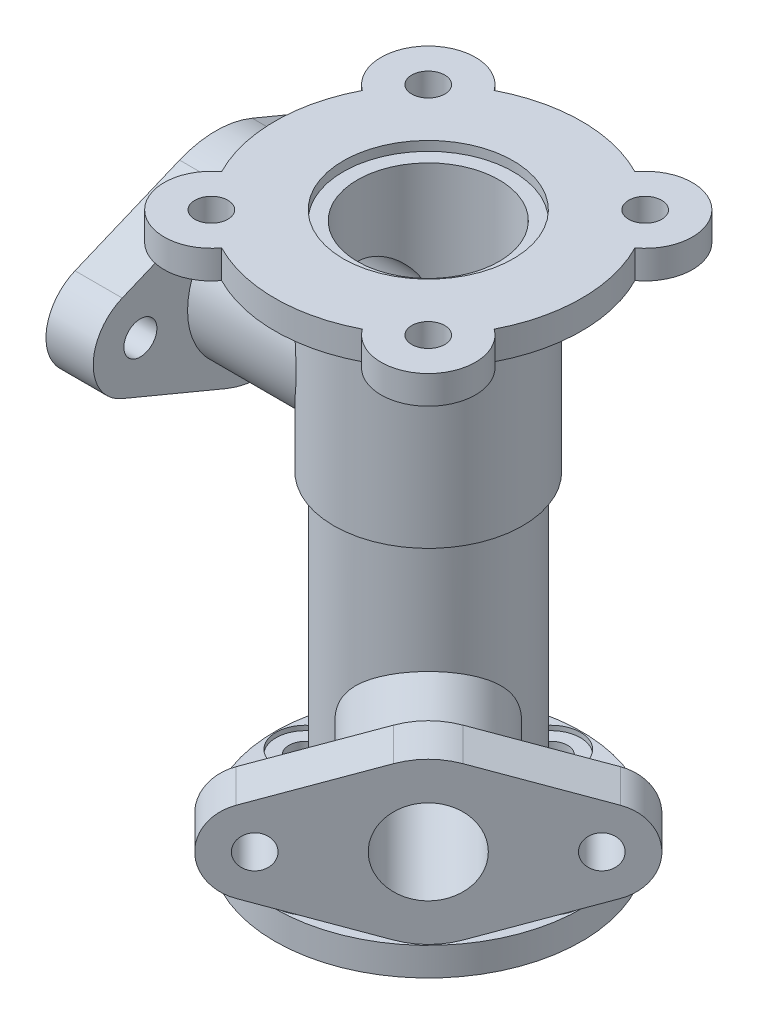
from build123d import *

# Parameters (mm, degrees)
SKETCH1_R           = 32.5
BOSS_EXTRUDE1_DEPTH = 6
SKETCH2_R           = 18
BOSS_EXTRUDE2_DEPTH = 64
SKETCH3_R           = 20
BOSS_EXTRUDE3_DEPTH = 48
BOSS_EXTRUDE4_START = -6
SKETCH4_R           = 32.5
SKETCH4_R_2         = 10
SKETCH4_R_3         = 20
BOSS_EXTRUDE4_DEPTH = 6
SKETCH5_R           = 16
BOSS_EXTRUDE5_DEPTH = 45
BOSS_EXTRUDE6_DEPTH = 10
SKETCH8_R           = 14
BOSS_EXTRUDE7_DEPTH = 45
BOSS_EXTRUDE8_DEPTH = 10
SKETCH10_R          = 13
CUT_EXTRUDE1_DEPTH  = 70
SKETCH11_R          = 9
CUT_EXTRUDE2_DEPTH  = 45
SKETCH12_R          = 11
CUT_EXTRUDE3_DEPTH  = 45
CUT_EXTRUDE4_START  = -2
SKETCH13_R          = 18
CUT_EXTRUDE4_DEPTH  = 2
SKETCH14_R          = 15
CUT_EXTRUDE5_DEPTH  = 36
SKETCH15_R          = 14
CUT_EXTRUDE6_DEPTH  = 3
SKETCH16_R          = 3.5
CUT_EXTRUDE7_DEPTH  = 20
SKETCH17_R          = 6.5
CUT_EXTRUDE8_DEPTH  = 1
SKETCH18_R          = 3.5
CUT_EXTRUDE9_DEPTH  = 10
SKETCH19_R          = 3.5
CUT_EXTRUDE10_DEPTH = 10
SKETCH20_R          = 3.5
CUT_EXTRUDE11_DEPTH = 20
SKETCH21_R          = 6.25
CUT_EXTRUDE12_DEPTH = 1
SKETCH22_R          = 10
CUT_EXTRUDE13_DEPTH = 50


with BuildPart() as part:
    # Sketch1 → Boss-Extrude1 (new body)
    with BuildSketch(Plane(origin=(0, 0, 0), x_dir=(1, 0, 0), z_dir=(0, 1, 0))):
        with Locations(Location((0, 0, 0), (0, 0, 270))):
            Circle(SKETCH1_R)
    extrude(amount=BOSS_EXTRUDE1_DEPTH)

    # Sketch2 → Boss-Extrude2 (add)
    with BuildSketch(Plane(origin=(0, 6, 0), x_dir=(1, 0, 0), z_dir=(0, 1, 0))):
        with Locations(Location((0, 0, 0), (0, 0, 270))):
            Circle(SKETCH2_R)
    extrude(amount=BOSS_EXTRUDE2_DEPTH)

    # Sketch3 → Boss-Extrude3 (add)
    with BuildSketch(Plane(origin=(0, 70, 0), x_dir=(1, 0, 0), z_dir=(0, 1, 0))):
        with Locations(Location((0, 0, 0), (0, 0, 270))):
            Circle(SKETCH3_R)
    extrude(amount=BOSS_EXTRUDE3_DEPTH)

    # Sketch4 → Boss-Extrude4 (add)
    # profile 1 of 18: a face of its own
    with BuildSketch(Plane(origin=(0, 118, 0), x_dir=(1, 0, 0), z_dir=(0, 1, 0)).offset(BOSS_EXTRUDE4_START)):
        with Locations(Location((0, 0, 0), (0, 0, 270))):
            Circle(SKETCH4_R)
    # profile 2 of 18: a face of its own
    with BuildSketch(Plane(origin=(0, 118, 0), x_dir=(1, 0, 0), z_dir=(0, 1, 0)).offset(BOSS_EXTRUDE4_START)):
        with Locations((22.980970389, 22.980970389)):
            Circle(SKETCH4_R_2)
    # profile 3 of 18: a face of its own
    with BuildSketch(Plane(origin=(0, 118, 0), x_dir=(1, 0, 0), z_dir=(0, 1, 0)).offset(BOSS_EXTRUDE4_START)):
        with Locations(Location((0, 0, 0), (0, 0, 270))):
            Circle(SKETCH4_R)
    # profile 4 of 18: a face of its own
    with BuildSketch(Plane(origin=(0, 118, 0), x_dir=(1, 0, 0), z_dir=(0, 1, 0)).offset(BOSS_EXTRUDE4_START)):
        with Locations((22.980970389, 22.980970389)):
            Circle(SKETCH4_R_2)
    # profile 5 of 18: a face of its own
    with BuildSketch(Plane(origin=(0, 118, 0), x_dir=(1, 0, 0), z_dir=(0, 1, 0)).offset(BOSS_EXTRUDE4_START)):
        with Locations((-22.980970389, 22.980970389)):
            Circle(SKETCH4_R_2)
    # profile 6 of 18: a face of its own
    with BuildSketch(Plane(origin=(0, 118, 0), x_dir=(1, 0, 0), z_dir=(0, 1, 0)).offset(BOSS_EXTRUDE4_START)):
        with Locations(Location((0, 0, 0), (0, 0, 270))):
            Circle(SKETCH4_R)
        with Locations(Location((0, 0, 0), (0, 0, 270))):
            Circle(SKETCH4_R_3, mode=Mode.SUBTRACT)
    # profile 7 of 18: a face of its own
    with BuildSketch(Plane(origin=(0, 118, 0), x_dir=(1, 0, 0), z_dir=(0, 1, 0)).offset(BOSS_EXTRUDE4_START)):
        with Locations((-22.980970389, -22.980970389)):
            Circle(SKETCH4_R_2)
    # profile 8 of 18: a face of its own
    with BuildSketch(Plane(origin=(0, 118, 0), x_dir=(1, 0, 0), z_dir=(0, 1, 0)).offset(BOSS_EXTRUDE4_START)):
        with Locations((22.980970389, -22.980970389)):
            Circle(SKETCH4_R_2)
    # profile 9 of 18: a face of its own
    with BuildSketch(Plane(origin=(0, 118, 0), x_dir=(1, 0, 0), z_dir=(0, 1, 0)).offset(BOSS_EXTRUDE4_START)):
        with Locations((22.980970389, 22.980970389)):
            Circle(SKETCH4_R_2)
    # profile 10 of 18: a face of its own
    with BuildSketch(Plane(origin=(0, 118, 0), x_dir=(1, 0, 0), z_dir=(0, 1, 0)).offset(BOSS_EXTRUDE4_START)):
        with Locations(Location((0, 0, 0), (0, 0, 270))):
            Circle(SKETCH4_R_3)
    # profile 11 of 18: a face of its own
    with BuildSketch(Plane(origin=(0, 118, 0), x_dir=(1, 0, 0), z_dir=(0, 1, 0)).offset(BOSS_EXTRUDE4_START)):
        with Locations(Location((0, 0, 0), (0, 0, 270))):
            Circle(SKETCH4_R)
    # profile 12 of 18: a face of its own
    with BuildSketch(Plane(origin=(0, 118, 0), x_dir=(1, 0, 0), z_dir=(0, 1, 0)).offset(BOSS_EXTRUDE4_START)):
        with Locations((22.980970389, -22.980970389)):
            Circle(SKETCH4_R_2)
    # profile 13 of 18: a face of its own
    with BuildSketch(Plane(origin=(0, 118, 0), x_dir=(1, 0, 0), z_dir=(0, 1, 0)).offset(BOSS_EXTRUDE4_START)):
        with Locations(Location((0, 0, 0), (0, 0, 270))):
            Circle(SKETCH4_R)
    # profile 14 of 18: a face of its own
    with BuildSketch(Plane(origin=(0, 118, 0), x_dir=(1, 0, 0), z_dir=(0, 1, 0)).offset(BOSS_EXTRUDE4_START)):
        with Locations((22.980970389, -22.980970389)):
            Circle(SKETCH4_R_2)
    # profile 15 of 18: a face of its own
    with BuildSketch(Plane(origin=(0, 118, 0), x_dir=(1, 0, 0), z_dir=(0, 1, 0)).offset(BOSS_EXTRUDE4_START)):
        with Locations(Location((0, 0, 0), (0, 0, 270))):
            Circle(SKETCH4_R)
    # profile 16 of 18: a face of its own
    with BuildSketch(Plane(origin=(0, 118, 0), x_dir=(1, 0, 0), z_dir=(0, 1, 0)).offset(BOSS_EXTRUDE4_START)):
        with Locations((-22.980970389, -22.980970389)):
            Circle(SKETCH4_R_2)
    # profile 17 of 18: a face of its own
    with BuildSketch(Plane(origin=(0, 118, 0), x_dir=(1, 0, 0), z_dir=(0, 1, 0)).offset(BOSS_EXTRUDE4_START)):
        with Locations(Location((0, 0, 0), (0, 0, 270))):
            Circle(SKETCH4_R)
    # profile 18 of 18: a face of its own
    with BuildSketch(Plane(origin=(0, 118, 0), x_dir=(1, 0, 0), z_dir=(0, 1, 0)).offset(BOSS_EXTRUDE4_START)):
        with Locations((-22.980970389, -22.980970389)):
            Circle(SKETCH4_R_2)
    extrude(amount=BOSS_EXTRUDE4_DEPTH)

    # Sketch5 → Boss-Extrude5 (add)
    with BuildSketch(Plane(origin=(0, 0, 0), x_dir=(0, 0, -1), z_dir=(1, 0, 0))):
        with Locations((0, 90)):
            Circle(SKETCH5_R)
    extrude(amount=-BOSS_EXTRUDE5_DEPTH)

    # Sketch6 → Boss-Extrude6 (add)
    with BuildSketch(Plane.ZY.offset(45)):
        with BuildLine():
            Line((7.692307692, 71.538461538), (29.846153846, 80.769230769))
            ThreePointArc((29.846153846, 80.769230769), (36, 90), (29.846153846, 99.230769231))
            Line((29.846153846, 99.230769231), (7.692307692, 108.461538462))
            ThreePointArc((7.692307692, 108.461538462), (0, 110), (-7.692307692, 108.461538462))
            Line((-7.692307692, 108.461538462), (-29.846153846, 99.230769231))
            ThreePointArc((-29.846153846, 99.230769231), (-36, 90), (-29.846153846, 80.769230769))
            Line((-29.846153846, 80.769230769), (-7.692307692, 71.538461538))
            ThreePointArc((-7.692307692, 71.538461538), (0, 70), (7.692307692, 71.538461538))
        make_face()
    extrude(amount=-BOSS_EXTRUDE6_DEPTH)

    # Sketch8 → Boss-Extrude7 (add)
    with BuildSketch(Plane(origin=(0, 0, 0), x_dir=(0, -1, 0), z_dir=(-0.7071067811865464, 0, -0.7071067811865488))):
        with Locations(Location((-32, 0, 0), (0, 0, 90))):
            Circle(SKETCH8_R)
    extrude(amount=-BOSS_EXTRUDE7_DEPTH)

    # Sketch9 → Boss-Extrude8 (add)
    with BuildSketch(Plane(origin=(31.819805153, 0, 31.819805153), x_dir=(0.7071067811865487, 0, -0.7071067811865465), z_dir=(0.7071067811865465, 0, 0.7071067811865487))):
        with BuildLine():
            Line((5.230769231, 15.824739469), (28.769230769, 23.436626778))
            ThreePointArc((28.769230769, 23.436626778), (35, 32), (28.769230769, 40.563373222))
            Line((28.769230769, 40.563373222), (5.230769231, 48.175260531))
            ThreePointArc((5.230769231, 48.175260531), (0, 49), (-5.230769231, 48.175260531))
            Line((-5.230769231, 48.175260531), (-28.769230769, 40.563373222))
            ThreePointArc((-28.769230769, 40.563373222), (-35, 32), (-28.769230769, 23.436626778))
            Line((-28.769230769, 23.436626778), (-5.230769231, 15.824739469))
            ThreePointArc((-5.230769231, 15.824739469), (0, 15), (5.230769231, 15.824739469))
        make_face()
    extrude(amount=-BOSS_EXTRUDE8_DEPTH)

    # Sketch10 → Cut-Extrude1 (cut)
    with BuildSketch(Plane.XZ):
        with Locations(Location((0, 0, 0), (0, 0, 270))):
            Circle(SKETCH10_R)
    extrude(amount=-CUT_EXTRUDE1_DEPTH, mode=Mode.SUBTRACT)

    # Sketch11 → Cut-Extrude2 (cut)
    with BuildSketch(Plane(origin=(31.819805153, 0, 31.819805153), x_dir=(0.7071067811865487, 0, -0.7071067811865465), z_dir=(0.7071067811865465, 0, 0.7071067811865487))):
        with Locations((0, 32)):
            Circle(SKETCH11_R)
    extrude(amount=-CUT_EXTRUDE2_DEPTH, mode=Mode.SUBTRACT)

    # Sketch12 → Cut-Extrude3 (cut)
    with BuildSketch(Plane.ZY.offset(45)):
        with Locations((0, 90)):
            Circle(SKETCH12_R)
    extrude(amount=-CUT_EXTRUDE3_DEPTH, mode=Mode.SUBTRACT)

    # Sketch13 → Cut-Extrude4 (cut)
    with BuildSketch(Plane(origin=(0, 118, 0), x_dir=(1, 0, 0), z_dir=(0, 1, 0)).offset(CUT_EXTRUDE4_START)):
        with Locations(Location((0, 0, 0), (0, 0, 270))):
            Circle(SKETCH13_R)
    extrude(amount=CUT_EXTRUDE4_DEPTH, mode=Mode.SUBTRACT)

    # Sketch14 → Cut-Extrude5 (cut)
    with BuildSketch(Plane(origin=(0, 116, 0), x_dir=(1, 0, 0), z_dir=(0, 1, 0))):
        with Locations(Location((0, 0, 0), (0, 0, 270))):
            Circle(SKETCH14_R)
    extrude(amount=-CUT_EXTRUDE5_DEPTH, mode=Mode.SUBTRACT)

    # Sketch15 → Cut-Extrude6 (cut)
    with BuildSketch(Plane(origin=(0, 80, 0), x_dir=(1, 0, 0), z_dir=(0, 1, 0))):
        with Locations(Location((0, 0, 0), (0, 0, 270))):
            Circle(SKETCH15_R)
    extrude(amount=-CUT_EXTRUDE6_DEPTH, mode=Mode.SUBTRACT)

    # Sketch16 → Cut-Extrude7 (cut)
    with BuildSketch(Plane(origin=(0, 118, 0), x_dir=(1, 0, 0), z_dir=(0, 1, 0))):
        with Locations(Location((22.980970389, 22.980970389, 0), (0, 0, 270))):
            Circle(SKETCH16_R)
        with Locations(Location((22.980970389, -22.980970389, 0), (0, 0, 270))):
            Circle(SKETCH16_R)
        with Locations(Location((-22.980970389, -22.980970389, 0), (0, 0, 270))):
            Circle(SKETCH16_R)
        with Locations(Location((-22.980970389, 22.980970389, 0), (0, 0, 270))):
            Circle(SKETCH16_R)
    extrude(amount=-CUT_EXTRUDE7_DEPTH, mode=Mode.SUBTRACT)

    # Sketch17 → Cut-Extrude8 (cut)
    with BuildSketch(Plane.XZ.offset(-112)):
        with Locations(Location((22.980970389, 22.980970389, 0), (0, 0, 270))):
            Circle(SKETCH17_R)
        with Locations(Location((22.980970389, -22.980970389, 0), (0, 0, 270))):
            Circle(SKETCH17_R)
        with Locations(Location((-22.980970389, -22.980970389, 0), (0, 0, 270))):
            Circle(SKETCH17_R)
        with Locations(Location((-22.980970389, 22.980970389, 0), (0, 0, 270))):
            Circle(SKETCH17_R)
    extrude(amount=-CUT_EXTRUDE8_DEPTH, mode=Mode.SUBTRACT)

    # Sketch18 → Cut-Extrude9 (cut)
    with BuildSketch(Plane(origin=(31.819805153, 0, 31.819805153), x_dir=(0.7071067811865487, 0, -0.7071067811865465), z_dir=(0.7071067811865465, 0, 0.7071067811865487))):
        with Locations((-26, 32)):
            Circle(SKETCH18_R)
        with Locations((26, 32)):
            Circle(SKETCH18_R)
    extrude(amount=-CUT_EXTRUDE9_DEPTH, mode=Mode.SUBTRACT)

    # Sketch19 → Cut-Extrude10 (cut)
    with BuildSketch(Plane.ZY.offset(45)):
        with Locations((26, 90)):
            Circle(SKETCH19_R)
        with Locations((-26, 90)):
            Circle(SKETCH19_R)
    extrude(amount=-CUT_EXTRUDE10_DEPTH, mode=Mode.SUBTRACT)

    # Sketch20 → Cut-Extrude11 (cut)
    with BuildSketch(Plane.XZ):
        with Locations(Location((0, -26, 0), (0, 0, 270))):
            Circle(SKETCH20_R)
        with Locations(Location((-26, 0, 0), (0, 0, 270))):
            Circle(SKETCH20_R)
        with Locations(Location((0, 26, 0), (0, 0, 270))):
            Circle(SKETCH20_R)
        with Locations(Location((26, 0, 0), (0, 0, 270))):
            Circle(SKETCH20_R)
    extrude(amount=-CUT_EXTRUDE11_DEPTH, mode=Mode.SUBTRACT)

    # Sketch21 → Cut-Extrude12 (cut)
    with BuildSketch(Plane(origin=(0, 6, 0), x_dir=(1, 0, 0), z_dir=(0, 1, 0))):
        with Locations(Location((-26, 0, 0), (0, 0, 270))):
            Circle(SKETCH21_R)
        with Locations(Location((0, 26, 0), (0, 0, 270))):
            Circle(SKETCH21_R)
        with Locations(Location((26, 0, 0), (0, 0, 270))):
            Circle(SKETCH21_R)
        with Locations(Location((0, -26, 0), (0, 0, 270))):
            Circle(SKETCH21_R)
    extrude(amount=-CUT_EXTRUDE12_DEPTH, mode=Mode.SUBTRACT)

    # Sketch22 → Cut-Extrude13 (cut)
    with BuildSketch(Plane(origin=(0, 77, 0), x_dir=(1, 0, 0), z_dir=(0, 1, 0))):
        with Locations(Location((0, 0, 0), (0, 0, 270))):
            Circle(SKETCH22_R)
    extrude(amount=-CUT_EXTRUDE13_DEPTH, mode=Mode.SUBTRACT)


solid = part.part
